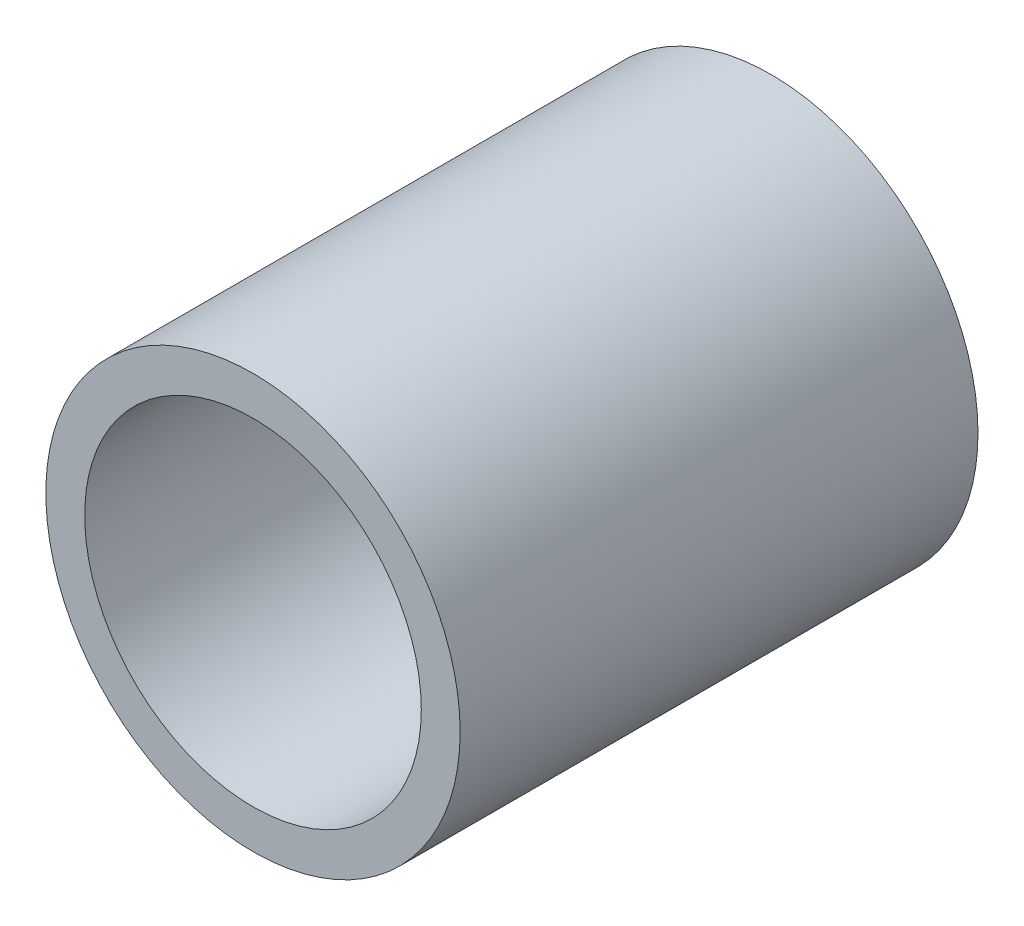
from build123d import *

# Parameters (mm, degrees)
SKETCH_1_R      = 16
SKETCH_1_R_2    = 13
EXTRUDE_1_DEPTH = 40


with BuildPart() as part:
    # 草图1 → 拉伸-薄壁1 (new body)
    with BuildSketch(Plane.XY):
        Circle(SKETCH_1_R)
        Circle(SKETCH_1_R_2, mode=Mode.SUBTRACT)
    extrude(amount=EXTRUDE_1_DEPTH)


solid = part.part
